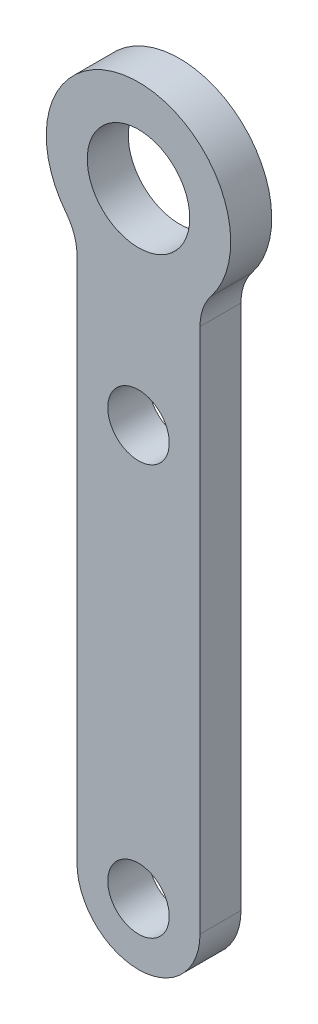
SolidWorks part; units mm, degrees
material "Plain Carbon Steel"
ref_plane "Front Plane" through (0, 0, 0) normal (0, 0, 1) x (1, 0, 0)
ref_plane "Top Plane" through (0, 0, 0) normal (0, 1, 0) x (1, 0, 0)
ref_plane "Right Plane" through (0, 0, 0) normal (1, 0, 0) x (0, 0, -1)
sketch "Sketch1" plane through (0, 0, 0) normal (0, 0, 1) x (1, 0, 0)
  line L0 (0, -1033.7506) -> (0, 50653.778) construction
  line L1 (-6, -60) -> (-6, -8.6603)
  line L2 (6, -60) -> (6, -8.6603)
  circle A0 centre (0, 0) radius 5
  circle A1 centre (0, -20) radius 3
  circle A2 centre (0, -60) radius 3
  arc A3 (-6, -60) -> (6, -60) centre (0, -60) ccw
  arc A4 (7.0714, -5.5673) -> (-7.0714, -5.5673) centre (0, 0) ccw
  arc A5 (-6, -8.6603) -> (-7.0714, -5.5673) centre (-11, -8.6603) ccw
  arc A6 (7.0714, -5.5673) -> (6, -8.6603) centre (11, -8.6603) ccw
  dimension "D1" = 6
  dimension "D2" = 10
  dimension "D3" = 9
  dimension "D4" = 12
  dimension "D7" = 5
  dimension "D8" = 5
  dimension "D5" = 20
  dimension "D6" = 40
extrude "Boss-Extrude1" add sketch "Sketch1" along normal blind 4
